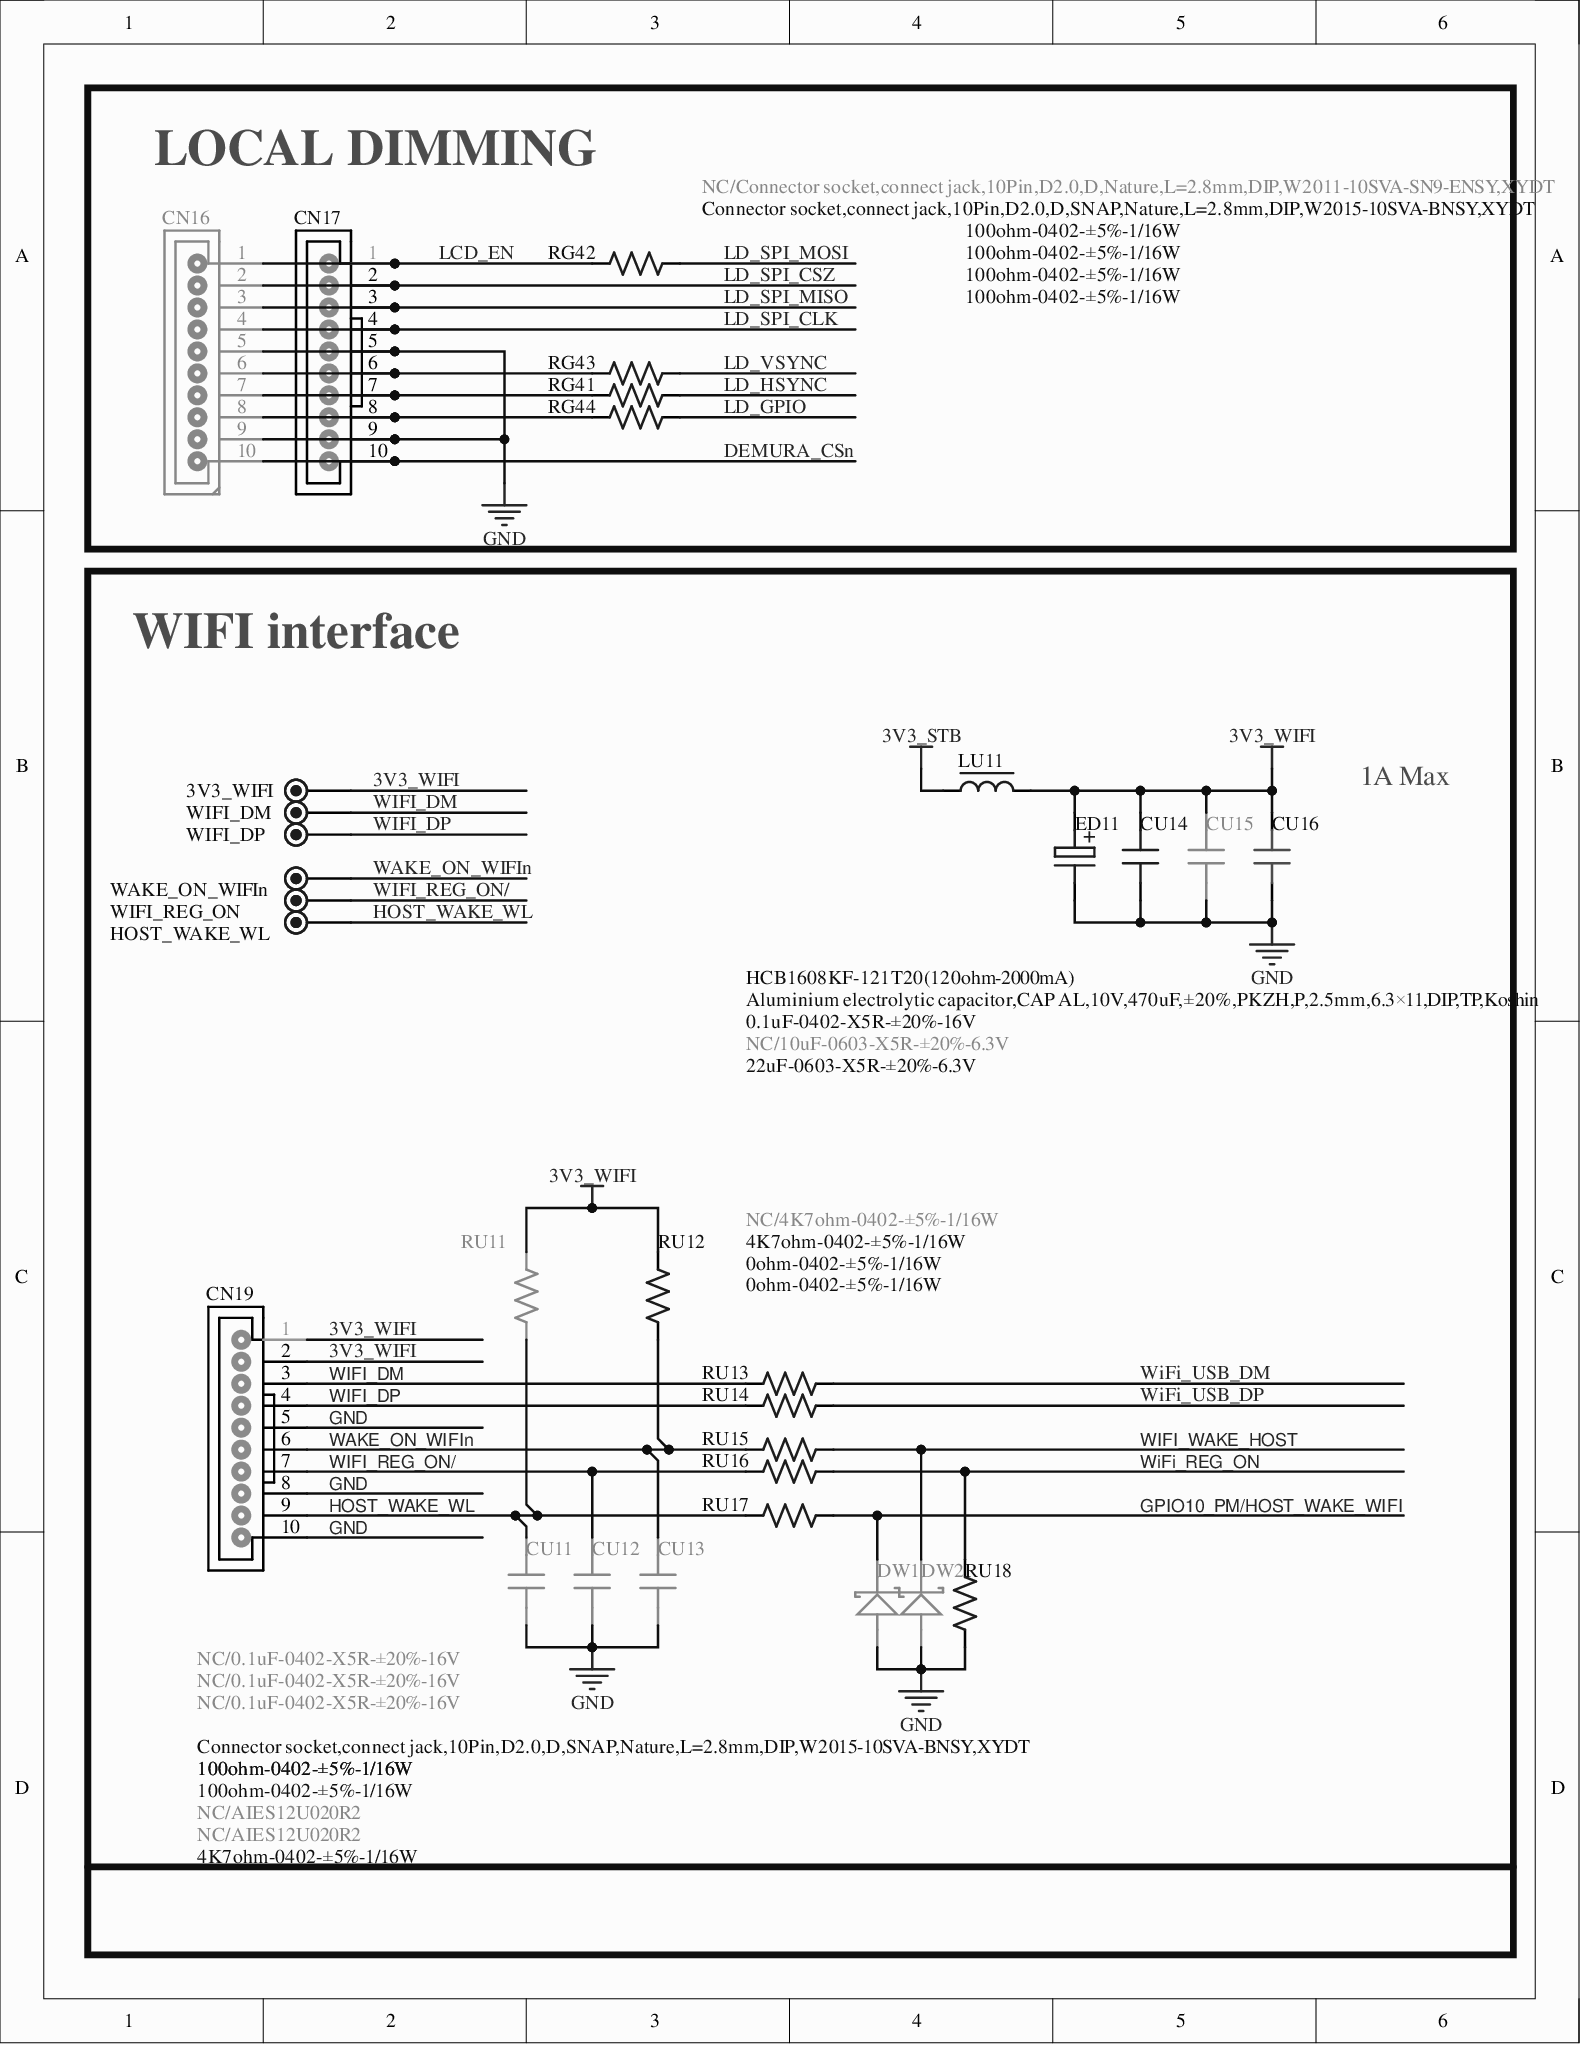
[diagram p0: MISC86290-19.SchDoc]
# Altium project MISC86290.PrjPcb (part 13 of 13)

## Sheet MISC86290-19.SchDoc
size 182 x 236 mm

### Parts
3V3_WIFI  TEST  [TP]  (value not drawn)
CN16  NC/Connector socket,connect jack,10Pin,D2.0,D,Nature,L=2.8mm,DIP,W2011-10SVA-SN9-ENSY,XYDT  [SIP10/2.0D-1]
CN17  Connector socket,connect jack,10Pin,D2.0,D,SNAP,Nature,L=2.8mm,DIP,W2015-10SVA-BNSY,XYDT  [SIP10/2.0D-4]
CN19  Connector socket,connect jack,10Pin,D2.0,D,SNAP,Nature,L=2.8mm,DIP,W2015-10SVA-BNSY,XYDT  [SIP10/2.0D-4]
CU11  NC/0.1uF-0402-X5R-±20%-16V  [C0402]
CU12  NC/0.1uF-0402-X5R-±20%-16V  [C0402]
CU13  NC/0.1uF-0402-X5R-±20%-16V  [C0402]
CU14  0.1uF-0402-X5R-±20%-16V  [C0402]
CU15  NC/10uF-0603-X5R-±20%-6.3V  [C0603]
CU16  22uF-0603-X5R-±20%-6.3V  [C0603]
DW1  NC/AIES12U020R2  [DIODE-S0402]
DW2  NC/AIES12U020R2  [DIODE-S0402]
ED11  Aluminium electrolytic capacitor,CAP AL,10V,470uF,±20%,PKZH,P,2.5mm,6.3×11,DIP,TP,Koshin  [EC(6.3*11)-V-2.5]
HOST_WAKE_WL  TEST  [TP]  (value not drawn)
LU11  HCB1608KF-121T20(120ohm-2000mA)  [L0603]
RG41  100ohm-0402-±5%-1/16W  [R0402]
RG42  100ohm-0402-±5%-1/16W  [R0402]
RG43  100ohm-0402-±5%-1/16W  [R0402]
RG44  100ohm-0402-±5%-1/16W  [R0402]
RU11  NC/4K7ohm-0402-±5%-1/16W  [R0402]
RU12  4K7ohm-0402-±5%-1/16W  [R0402]
RU13  0ohm-0402-±5%-1/16W  [R0402]
RU14  0ohm-0402-±5%-1/16W  [R0402]
RU15  100ohm-0402-±5%-1/16W  [R0402]
RU16  100ohm-0402-±5%-1/16W  [R0402]
RU17  100ohm-0402-±5%-1/16W  [R0402]
RU18  4K7ohm-0402-±5%-1/16W  [R0402]
WAKE_ON_WIFIn  TEST  [TP]  (value not drawn)
WIFI_DM  TEST  [TP]  (value not drawn)
WIFI_DP  TEST  [TP]  (value not drawn)
WIFI_REG_ON  TEST  [TP]  (value not drawn)

### Blocks framed on the sheet
LOCAL DIMMING: CN16 CN17 RG41-RG44
WIFI interface: 3V3_WIFI CN19 CU11-CU16 DW1 DW2 ED11 HOST_WAKE_WL LU11 RU11-RU18 WAKE_ON_WIFIn WIFI_DM WIFI_DP WIFI_REG_ON

### Nets
3V3_STB: LU11.1
3V3_WIFI: 3V3_WIFI.1 CN19.1 CN19.2 CU14.2 CU15.2 CU16.2 ED11.1 LU11.2 RU11.2 RU12.2
GND: CN16.5 CN16.9 CN17.5 CN17.9 CN19.5 CN19.8 CN19.10 CU11.2 CU12.2 CU13.2 CU14.1 CU15.1 CU16.1 DW1.A DW2.A ED11.2 RU18.1
DEMURA_CSn: CN16.10 CN17.10
GPIO10_PM/HOST_WAKE_WIFI: DW1.K RU17.2
HOST_WAKE_WL: CN19.9 CU11.1 HOST_WAKE_WL.1 RU11.1 RU17.1
LCD_EN: CN16.1 CN17.1 RG42.1
LD_GPIO: RG44.2
LD_HSYNC: RG41.2
LD_SPI_CLK: CN16.4 CN17.4
LD_SPI_CSZ: CN16.2 CN17.2
LD_SPI_MISO: CN16.3 CN17.3
LD_SPI_MOSI: RG42.2
LD_VSYNC: RG43.2
WAKE_ON_WIFIn: CN19.6 CU13.1 RU12.1 RU15.1 WAKE_ON_WIFIn.1
WIFI_DM: CN19.3 RU13.1 WIFI_DM.1
WIFI_DP: CN19.4 RU14.1 WIFI_DP.1
WiFi_REG_ON: RU16.2 RU18.2
WIFI_REG_ON/: CN19.7 CU12.1 RU16.1 WIFI_REG_ON.1
WiFi_USB_DM: RU13.2
WiFi_USB_DP: RU14.2
WIFI_WAKE_HOST: DW2.K RU15.2
NetCN16_6: CN16.6 CN17.6 RG43.1
NetCN16_7: CN16.7 CN17.7 RG41.1
NetCN16_8: CN16.8 CN17.8 RG44.1

### Notes on the sheet
- 1A Max

### Library data of the parts
CN16 = XXX.XXX.0000613-DHMI: Connector socket,connect jack,10Pin,D2.0,D,L=2.8mm,DIP,CNJST-DHMI
CN17 = XXX.XXX.0000646-DHMI: Connector socket,connect jack,10Pin,D2.0,D,SNAP,L=2.8mm,DIP,CNJST-DHMI
CN19 = 10PIN-2.0-D-H-G-带扣-J-DHMI
CU11-CU13 = 0.1uF-0402-X7R-±10%-16V-D
CU14 = 0.1uF-0402-Y5V-+80%-20%-16V-D
CU15 CU16 = 22uF-0603-X5R-±20%-6.3V-D
DW1 DW2 = AIES12U020R2-D
ED11 = 470uF-10V-±20%-6.3×11-105℃-黑底白字-编带-F=2.5-XF-DHAI: Electrolytic
LU11 = HCB1608KF-121T20(120ohm-2000mA)-D
RG41-RG44 RU13-RU17 = 0ohm-0402-±5%-1/16W-D
RU11 RU12 RU18 = 4K7ohm-0402-±5%-1/16W-D

## Nets that join several sheets
0.95V_VDDC: MISC86290-6 (10 pins), MISC86290-7 (30 pins)
0.95V_VDDCPU: MISC86290-6 (7 pins), MISC86290-7 (22 pins)
1V5_DDR: MISC86290-6 (8 pins), MISC86290-7 (31 pins), MISC86290-11 (79 pins)
3V3_M: MISC86290-6 (10 pins), MISC86290-7 (20 pins), MISC86290-9 (11 pins), MISC86290-10 (13 pins), MISC86290-12 (9 pins), MISC86290-14 (LO2.2 LO3.2 RO46.2 RO47.2), MISC86290-16 (RU5.1), MISC86290-17 (6 pins), MISC86290-18 (RT7.2 RT40.1)
3V3_STB: MISC86290-6 (20 pins), MISC86290-7 (15 pins), MISC86290-9 (11 pins), MISC86290-13 (6 pins), MISC86290-19 (LU11.1)
3V3_Tun: MISC86290-6 (5 pins), MISC86290-14 (RO23.1 RO26.1), MISC86290-18 (CT3.2 CT33.2 FT1.1 RT40.2)
5V_M: MISC86290-6 (24 pins), MISC86290-13 (RK10.2), MISC86290-14 (RO3.1 RO19.2 RO41.2), MISC86290-16 (CU3.2 CU4.2 FU1.1 UH3.5)
12V: MISC86290-6 (21 pins), MISC86290-9 (R120.2), MISC86290-17 (RA22.1 RA24.2)
AMP_VCC: MISC86290-6 (CNP2.1 CNP2.2), MISC86290-17 (13 pins)
GND: MISC86290-2 (36 pins), MISC86290-3 (C200.2 C201.1 C202.1 C205.1), MISC86290-6 (94 pins), MISC86290-7 (61 pins), MISC86290-8 (333 pins), MISC86290-9 (39 pins), MISC86290-10 (23 pins), MISC86290-11 (106 pins), MISC86290-12 (65 pins), MISC86290-13 (12 pins), MISC86290-14 (67 pins), MISC86290-15 (85 pins), MISC86290-16 (33 pins), MISC86290-17 (62 pins), MISC86290-18 (48 pins), MISC86290-19 (17 pins)
MOD_1V2: MISC86290-6 (5 pins), MISC86290-7 (C25.2 C26.1 U1.AK23)
VCC_Panel: MISC86290-6 (9 pins), MISC86290-12 (36 pins)
AMP_MUTEn: MISC86290-10 (U1.AH23), MISC86290-17 (CNA5.9 RA9.2 RA20.2)
AMP_RSTn: MISC86290-10 (U1.AH22), MISC86290-17 (CNA5.10 RA11.2 RA21.1 RA34.2)
AUBCK_OUT: MISC86290-9 (U1.C4), MISC86290-17 (CNA5.2 RA3.1)
AUMCK_OUT: MISC86290-9 (U1.E5), MISC86290-17 (CNA5.1 RA4.1)
AUSD_OUT: MISC86290-9 (U1.C5), MISC86290-17 (CNA5.3 RA1.1)
AUWS_OUT: MISC86290-9 (U1.B5), MISC86290-17 (CNA5.4 RA2.1)
DEMURA_CSn: MISC86290-9 (R125.2), MISC86290-19 (CN16.10 CN17.10)
FRC_ALIVE: MISC86290-9 (R204.2), MISC86290-10 (U1.V27)
FRC_DCD_RCR: MISC86290-9 (R205.2), MISC86290-10 (U1.W27)
FRC_RESETn: MISC86290-9 (R203.2), MISC86290-10 (U1.AA27)
GPIO10_PM/HOST_WAKE_WIFI: MISC86290-9 (R152.2 U1.M5), MISC86290-19 (DW1.K RU17.2)
HDMI-ARC_IC: MISC86290-9 (U1.AA4), MISC86290-15 (CH7.2)
HDMI-CEC_IC: MISC86290-9 (U1.Y4), MISC86290-15 (RH17.2)
HDMIA-Detect: MISC86290-9 (U1.Y5), MISC86290-15 (RH4.1)
HDMIA-HOTPLUG: MISC86290-9 (U1.W5), MISC86290-15 (RH1.1)
HDMIA-RX0N: MISC86290-9 (U1.W1), MISC86290-15 (AVH1.9 UH2.2 UH2.7)
HDMIA-RX0P: MISC86290-9 (U1.W2), MISC86290-15 (AVH1.7 UH2.1 UH2.8)
HDMIA-RX1N: MISC86290-9 (U1.Y3), MISC86290-15 (AVH1.6 UH1.4 UH1.5)
HDMIA-RX1P: MISC86290-9 (U1.Y2), MISC86290-15 (AVH1.4 UH1.3 UH1.6)
HDMIA-RX2N: MISC86290-9 (U1.AA3), MISC86290-15 (AVH1.3 UH1.2 UH1.7)
HDMIA-RX2P: MISC86290-9 (U1.AA2), MISC86290-15 (AVH1.1 UH1.1 UH1.8)
HDMIA-RXCKN: MISC86290-9 (U1.V1), MISC86290-15 (AVH1.12 UH2.4 UH2.5)
HDMIA-RXCKP: MISC86290-9 (U1.W3), MISC86290-15 (AVH1.10 UH2.3 UH2.6)
HDMIA-SCL_IC: MISC86290-9 (U1.AA5), MISC86290-15 (RH5.2)
HDMIA-SDA_IC: MISC86290-9 (U1.Y6), MISC86290-15 (RH6.2)
HDMIB-Detect: MISC86290-9 (U1.U4), MISC86290-15 (RH12.1)
HDMIB-HOTPLUG: MISC86290-9 (U1.U5), MISC86290-15 (RH11.1)
HDMIB-RX0N: MISC86290-9 (U1.R2), MISC86290-15 (AVH2.9 UH12.2 UH12.7)
HDMIB-RX0P: MISC86290-9 (U1.T3), MISC86290-15 (AVH2.7 UH12.1 UH12.8)
HDMIB-RX1N: MISC86290-9 (U1.T2), MISC86290-15 (AVH2.6 UH11.4 UH11.5)
HDMIB-RX1P: MISC86290-9 (U1.U3), MISC86290-15 (AVH2.4 UH11.3 UH11.6)
HDMIB-RX2N: MISC86290-9 (U1.U2), MISC86290-15 (AVH2.3 UH11.2 UH11.7)
HDMIB-RX2P: MISC86290-9 (U1.V3), MISC86290-15 (AVH2.1 UH11.1 UH11.8)
HDMIB-RXCKN: MISC86290-9 (U1.R3), MISC86290-15 (AVH2.12 UH12.4 UH12.5)
HDMIB-RXCKP: MISC86290-9 (U1.R1), MISC86290-15 (AVH2.10 UH12.3 UH12.6)
HDMIB-SCL_IC: MISC86290-9 (U1.W6), MISC86290-15 (RH15.2)
HDMIB-SDA_IC: MISC86290-9 (U1.U6), MISC86290-15 (RH16.2)
HDMIC-Detect: MISC86290-9 (U1.U7), MISC86290-15 (DH37.K RH32.1)
HDMIC-HOTPLUG: MISC86290-9 (U1.N4), MISC86290-15 (RH31.1)
HDMIC-RX0N: MISC86290-9 (U1.H2), MISC86290-15 (AVH4.9 UH32.2 UH32.7)
HDMIC-RX0P: MISC86290-9 (U1.J3), MISC86290-15 (AVH4.7 UH32.1 UH32.8)
HDMIC-RX1N: MISC86290-9 (U1.J2), MISC86290-15 (AVH4.6 UH31.4 UH31.5)
HDMIC-RX1P: MISC86290-9 (U1.K3), MISC86290-15 (AVH4.4 UH31.3 UH31.6)
HDMIC-RX2N: MISC86290-9 (U1.K2), MISC86290-15 (AVH4.3 UH31.2 UH31.7)
HDMIC-RX2P: MISC86290-9 (U1.K1), MISC86290-15 (AVH4.1 UH31.1 UH31.8)
HDMIC-RXCKN: MISC86290-9 (U1.G2), MISC86290-15 (AVH4.12 UH32.4 UH32.5)
HDMIC-RXCKP: MISC86290-9 (U1.H3), MISC86290-15 (AVH4.10 UH32.3 UH32.6)
HDMIC-SCL_IC: MISC86290-9 (U1.P5), MISC86290-15 (RH35.2)
HDMIC-SDA_IC: MISC86290-9 (U1.P6), MISC86290-15 (RH36.2)
HDMID-Detect: MISC86290-9 (U1.T6), MISC86290-15 (RH22.1)
HDMID-HOTPLUG: MISC86290-9 (U1.P7), MISC86290-15 (RH21.1)
HDMID-RX0N: MISC86290-9 (U1.M3), MISC86290-15 (AVH3.9 UH22.2 UH22.7)
HDMID-RX0P: MISC86290-9 (U1.M2), MISC86290-15 (AVH3.7 UH22.1 UH22.8)
HDMID-RX1N: MISC86290-9 (U1.N3), MISC86290-15 (AVH3.6 UH21.4 UH21.5)
HDMID-RX1P: MISC86290-9 (U1.N2), MISC86290-15 (AVH3.4 UH21.3 UH21.6)
HDMID-RX2N: MISC86290-9 (U1.P3), MISC86290-15 (AVH3.3 UH21.2 UH21.7)
HDMID-RX2P: MISC86290-9 (U1.P2), MISC86290-15 (AVH3.1 UH21.1 UH21.8)
HDMID-RXCKN: MISC86290-9 (U1.L1), MISC86290-15 (AVH3.12 UH22.4 UH22.5)
HDMID-RXCKP: MISC86290-9 (U1.L2), MISC86290-15 (AVH3.10 UH22.3 UH22.6)
HDMID-SCL_IC: MISC86290-9 (U1.R5), MISC86290-15 (RH25.2)
HDMID-SDA_IC: MISC86290-9 (U1.N6), MISC86290-15 (RH26.2)
HP_AU_LOUT: MISC86290-9 (U1.AG5), MISC86290-14 (CO12.2 CO14.2)
HP_AU_ROUT: MISC86290-9 (U1.AG4), MISC86290-14 (CO11.2 CO13.2)
HP_DET: MISC86290-10 (U1.AB26), MISC86290-14 (CO24.2 HP_DET.1 RO22.2 RO28.2)
HP_MUTEn: MISC86290-10 (U1.AC26), MISC86290-14 (RO29.1 RO30.2)
I2S_OUT_SD1: MISC86290-9 (R135.2), MISC86290-17 (CNA5.5)
I2S_OUT_SD2: MISC86290-9 (R136.2), MISC86290-17 (CNA5.6)
IR_IN_IC: MISC86290-9 (U1.K5), MISC86290-13 (CK1.2 RK2.2)
LD_GPIO: MISC86290-10 (U1.Y25), MISC86290-19 (RG44.2)
LD_HSYNC: MISC86290-9 (R130.1 U1.T28), MISC86290-19 (RG41.2)
LD_SPI_CLK: MISC86290-9 (R129.2), MISC86290-19 (CN16.4 CN17.4)
LD_SPI_CSZ: MISC86290-9 (R127.2), MISC86290-19 (CN16.2 CN17.2)
LD_SPI_MISO: MISC86290-9 (R126.2), MISC86290-19 (CN16.3 CN17.3)
LD_SPI_MOSI: MISC86290-9 (R128.2), MISC86290-19 (RG42.2)
LD_VSYNC: MISC86290-9 (U1.L28), MISC86290-19 (RG43.2)
LED_OUT_IC: MISC86290-9 (U1.D2), MISC86290-13 (RK13.1 RK14.1 RK15.2)
LINEOUT_L: MISC86290-9 (RO51.2 RO53.2), MISC86290-14 (CO32.2 CO34.1)
LINEOUT_MUTEn: MISC86290-10 (U1.AB27), MISC86290-14 (RO44.1 RO45.2)
LINEOUT_R: MISC86290-9 (RO52.2 RO54.2), MISC86290-14 (CO31.2 CO33.1)
LOG_RX: MISC86290-9 (R72.2), MISC86290-10 (U1.AE4), MISC86290-15 (RH38.2)
LOG_TX: MISC86290-9 (R73.2), MISC86290-10 (U1.AF3), MISC86290-15 (RH37.2)
MI2C_SCL: MISC86290-9 (D5.K R122.1 R200.1), MISC86290-12 (QW2.D RW395.2), MISC86290-13 (RK40.1), MISC86290-17 (CNA5.13 RA14.1)
MI2C_SDA: MISC86290-9 (D4.K R124.1 R201.1), MISC86290-12 (QW1.D RW393.2), MISC86290-13 (RK41.1), MISC86290-17 (CNA5.14 RA12.1)
PANEL_ISOLATEn: MISC86290-10 (U1.AG23), MISC86290-12 (RW5.1)
PHY_RX_N: MISC86290-9 (U1.A2), MISC86290-16 (RE23.1 UE2.1 UE2.8)
PHY_RX_P: MISC86290-9 (U1.B3), MISC86290-16 (RE22.1 UE2.2 UE2.7)
PHY_TX_N: MISC86290-9 (U1.B2), MISC86290-16 (RE21.1 UE2.3 UE2.6)
PHY_TX_P: MISC86290-9 (U1.B1), MISC86290-16 (RE20.1 UE2.4 UE2.5)
RCA_AU_LIN: MISC86290-9 (U1.AF2), MISC86290-14 (CI4.2)
RCA_AU_RIN: MISC86290-9 (U1.AF1), MISC86290-14 (CI6.2)
RCA_CVBSIN: MISC86290-9 (U1.AC6), MISC86290-14 (CI2.2)
RST_BTNn_LATCH: MISC86290-9 (DR5.K RR14.2), MISC86290-10 (U1.AJ20)
SAR0: MISC86290-9 (U1.D3), MISC86290-13 (RK26.1)
SAR1: MISC86290-9 (U1.C2), MISC86290-13 (RK33.1)
SOC_BL_ADIM: MISC86290-6 (RG33.1), MISC86290-9 (R130.2)
SOC_BL_ON: MISC86290-6 (DG1.K RG2.2 RG5.2 RG6.1), MISC86290-10 (U1.AH20)
SOC_BL_PDIM: MISC86290-6 (DG11.K RG11.2 RG15.2 RG16.1), MISC86290-9 (U1.L29)
SOC_BOOSTER: MISC86290-6 (RG32.1), MISC86290-10 (U1.AH21)
SOC_PANEL_ON: MISC86290-6 (RM11.1 RM12.2), MISC86290-10 (U1.AG26)
SOC_PS_ON: MISC86290-6 (RD1.1 RM1.1 RP1.1 RP8.2), MISC86290-9 (U1.M6)
SPDIF_OUT_IC: MISC86290-9 (U1.K6), MISC86290-14 (CO3.2 RO1.1)
TUNER_AGC_IC: MISC86290-10 (U1.AJ2), MISC86290-18 (RT1.2 RT7.1)
TUNER_IFM_IC: MISC86290-10 (U1.AK4), MISC86290-18 (CT32.2)
TUNER_IFP_IC: MISC86290-10 (U1.AJ4), MISC86290-18 (CT27.1)
TUNER_SCL_IC: MISC86290-10 (U1.AE7), MISC86290-18 (DT2.K RT6.1 RT8.2)
TUNER_SDA_IC: MISC86290-10 (U1.AF7), MISC86290-18 (DT3.K RT2.2 RT5.1)
USB_EN: MISC86290-9 (U1.K4), MISC86290-16 (RU10.2)
USB_OCn: MISC86290-10 (U1.AJ19), MISC86290-16 (RU9.1)
USB_P1_DM: MISC86290-9 (U1.E2), MISC86290-16 (RU1.1)
USB_P1_DP: MISC86290-9 (U1.F3), MISC86290-16 (RU2.1)
USB_P2_DM: MISC86290-9 (U1.AJ6), MISC86290-16 (RU7.1)
USB_P2_DP: MISC86290-9 (U1.AH7), MISC86290-16 (RU8.1)
VBY0N: MISC86290-9 (U1.AA30), MISC86290-12 (CW244.1)
VBY0P: MISC86290-9 (U1.AA29), MISC86290-12 (CW245.1)
VBY1N: MISC86290-9 (U1.AA28), MISC86290-12 (CW246.1)
VBY1P: MISC86290-9 (U1.AB29), MISC86290-12 (CW247.1)
VBY2N: MISC86290-9 (U1.AC29), MISC86290-12 (CW248.1)
VBY2P: MISC86290-9 (U1.AC28), MISC86290-12 (CW249.1)
VBY3N: MISC86290-9 (U1.AD29), MISC86290-12 (CW250.1)
VBY3P: MISC86290-9 (U1.AD30), MISC86290-12 (CW251.1)
VBY4N: MISC86290-9 (U1.AE30), MISC86290-12 (CW252.1)
VBY4P: MISC86290-9 (U1.AE29), MISC86290-12 (CW253.1)
VBY5N: MISC86290-9 (U1.AE28), MISC86290-12 (CW254.1)
VBY5P: MISC86290-9 (U1.AF29), MISC86290-12 (CW255.1)
VBY6N: MISC86290-9 (U1.AG29), MISC86290-12 (CW256.1)
VBY6P: MISC86290-9 (U1.AG28), MISC86290-12 (CW257.1)
VBY7N: MISC86290-9 (U1.AH29), MISC86290-12 (CW258.1)
VBY7P: MISC86290-9 (U1.AH30), MISC86290-12 (CW259.1)
VBY_HTPDn: MISC86290-9 (U1.AH25), MISC86290-12 (RW9.2 RW11.2)
VBY_LOCKn: MISC86290-9 (U1.AJ25), MISC86290-12 (RW8.2 RW10.2)
VDDC_PGOOD: MISC86290-6 (UD4.4), MISC86290-9 (RR7.2)
VDDCPU_PGOOD: MISC86290-6 (UD5.5), MISC86290-9 (RR6.2)
VID0: MISC86290-6 (RD37.1), MISC86290-9 (U1.AG6)
VID1: MISC86290-6 (RD35.1), MISC86290-9 (U1.AG7)
VID2: MISC86290-6 (RD58.1), MISC86290-9 (U1.AE5)
VID3: MISC86290-6 (RD59.1), MISC86290-9 (U1.AD6)
WiFi_REG_ON: MISC86290-9 (U1.AJ8), MISC86290-19 (RU16.2 RU18.2)
WiFi_USB_DM: MISC86290-9 (U1.AJ7), MISC86290-19 (RU13.2)
WiFi_USB_DP: MISC86290-9 (U1.AH8), MISC86290-19 (RU14.2)
WIFI_WAKE_HOST: MISC86290-9 (U1.AG8), MISC86290-19 (DW2.K RU15.2)